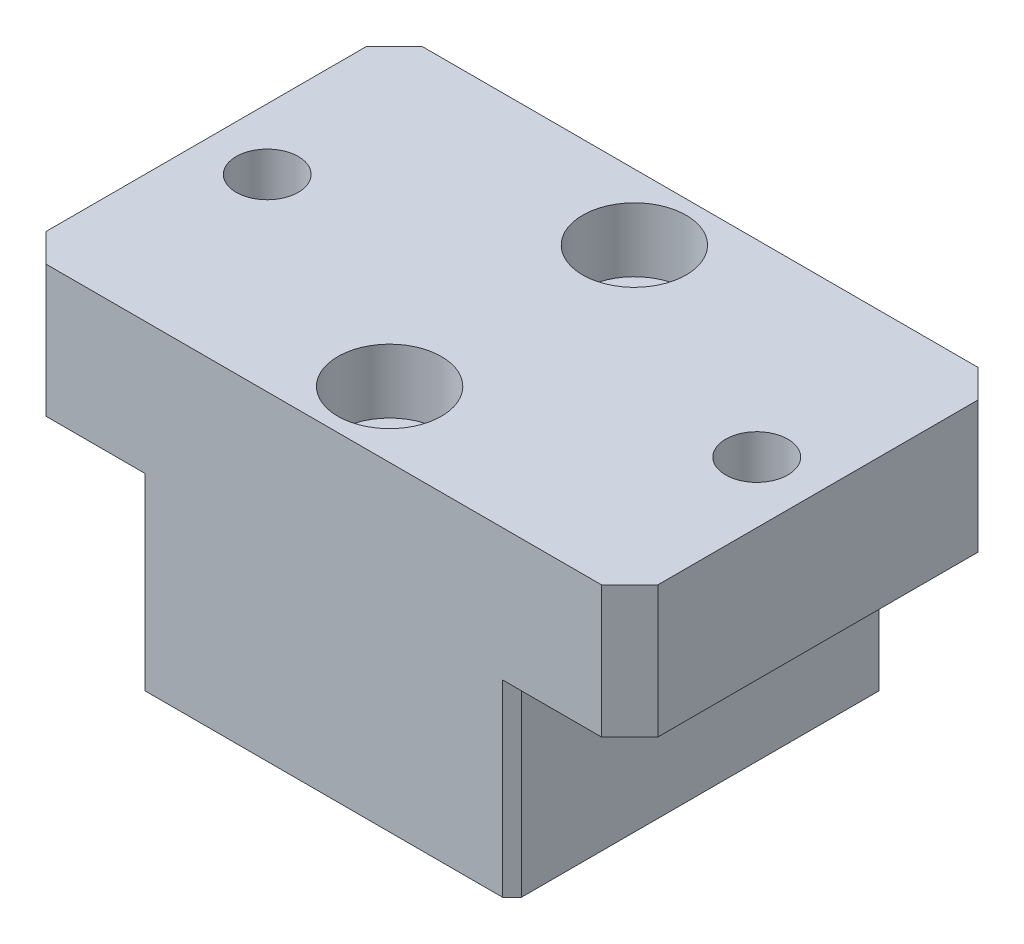
from build123d import *

# Parameters (mm, degrees)
SKETCH_1_W                  = 65
SKETCH_1_H                  = 40
EXTRUDE_1_DEPTH             = 17
HOLE_WIZARD_2_D             = 6.6
HOLE_WIZARD_2_CBORE_D       = 11
HOLE_WIZARD_2_CBORE_DEPTH   = 6.8
CHAMFER_1_SIZE              = 3
SKETCH_6_OUTSIDE_W          = 83.71
SKETCH_6_OUTSIDE_H          = 58.71
SKETCH_6_OUTSIDE_W_2        = 40
SKETCH_6_OUTSIDE_H_2        = 40
CUT_EXTRUDE_1_DEPTH         = 20
HOLE_WIZARD_2_2_D           = 6.6
HOLE_WIZARD_2_2_CBORE_D     = 11
HOLE_WIZARD_2_2_CBORE_DEPTH = 5
CHAMFER_2_SIZE              = 1


with BuildPart() as part:
    # 草图1 → 凸台-拉伸1 (new, symmetric)
    with BuildSketch(Plane(origin=(0, 0, 0), x_dir=(1, 0, 0), z_dir=(0, 1, 0))):
        Rectangle(SKETCH_1_W, SKETCH_1_H)
    extrude(amount=EXTRUDE_1_DEPTH, both=True)

    # Hole Wizard 2 (through all)
    with Locations(Plane(origin=(0, 17, 0), x_dir=(1, 0, 0), z_dir=(0, 1, 0))):
        with Locations((0, -13), (0, 13)):
            CounterBoreHole(HOLE_WIZARD_2_D / 2, HOLE_WIZARD_2_CBORE_D / 2, HOLE_WIZARD_2_CBORE_DEPTH)

    # 倒角1
    chamfer_1_edges = [part.edges().sort_by_distance(p)[0] for p in [
        (32.5, 0, 20),
        (-32.5, 0, 20),
        (-32.5, 0, -20),
        (32.5, 0, -20),
    ]]
    chamfer(chamfer_1_edges, length=CHAMFER_1_SIZE)

    # 草图6 outside → 切除-拉伸1 (cut)
    with BuildSketch(Plane.XZ.offset(17)):
        Rectangle(SKETCH_6_OUTSIDE_W, SKETCH_6_OUTSIDE_H)
        Rectangle(SKETCH_6_OUTSIDE_W_2, SKETCH_6_OUTSIDE_H_2, mode=Mode.SUBTRACT)
    extrude(amount=-CUT_EXTRUDE_1_DEPTH, mode=Mode.SUBTRACT)

    # Hole Wizard 2 2 (through all)
    with Locations(Plane.XZ.offset(-3)):
        with Locations((26, 0), (-26, 0)):
            CounterBoreHole(HOLE_WIZARD_2_2_D / 2, HOLE_WIZARD_2_2_CBORE_D / 2, HOLE_WIZARD_2_2_CBORE_DEPTH)

    # 倒角2
    chamfer_2_edges = [part.edges().sort_by_distance(p)[0] for p in [
        (-20, -7, 20),
        (20, -7, 20),
        (20, -7, -20),
        (-20, -7, -20),
    ]]
    chamfer(chamfer_2_edges, length=CHAMFER_2_SIZE)


solid = part.part
